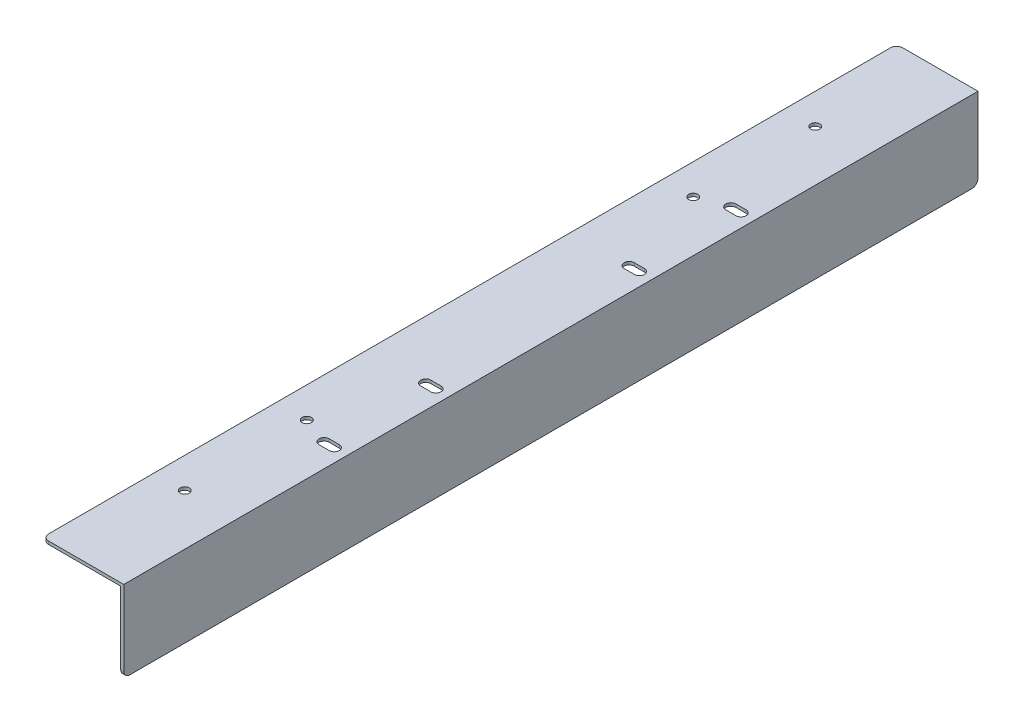
from build123d import *

# Parameters (mm, degrees)
SKETCH_1_W          = 420
SKETCH_1_H          = 40
EXTRUDE_1_DEPTH     = 1.5
SKETCH_2_W          = 420
SKETCH_2_H          = 1.5
EXTRUDE_2_DEPTH     = 40
FILLET_1_R          = 3
SKETCH_3_R          = 2.25
CUT_EXTRUDE_1_DEPTH = 10
SKETCH_6_R          = 2.25
CUT_EXTRUDE_2_DEPTH = 10
CUT_EXTRUDE_3_DEPTH = 218.214755484
CUT_EXTRUDE_4_DEPTH = 218.214755484


with BuildPart() as part:
    # 草图1 → 凸台-拉伸1 (new body)
    with BuildSketch(Plane(origin=(0, 0, 0), x_dir=(0, 0, -1), z_dir=(1, 0, 0))):
        Rectangle(SKETCH_1_W, SKETCH_1_H)
    extrude(amount=EXTRUDE_1_DEPTH)

    # 草图2 → 凸台-拉伸2 (add)
    with BuildSketch(Plane(origin=(1.5, 0, 0), x_dir=(0, 0, -1), z_dir=(1, 0, 0))):
        with Locations((0, 19.25)):
            Rectangle(SKETCH_2_W, SKETCH_2_H)
    extrude(amount=-EXTRUDE_2_DEPTH)

    # 圆角1
    fillet_1_edges = [part.edges().sort_by_distance(p)[0] for p in [
        (-38.5, 19.25, 210),
        (-38.5, 19.25, -210),
        (0.75, -20, -210),
        (0.75, -20, 210),
    ]]
    fillet(fillet_1_edges, radius=FILLET_1_R)

    # 草图3 → 切除-拉伸1 (cut)
    with BuildSketch(Plane(origin=(0, 20, 0), x_dir=(1, 0, 0), z_dir=(0, 1, 0))):
        with Locations(Location((-23.5, -95, 0), (0, 0, 270))):
            Circle(SKETCH_3_R)
        with Locations(Location((-23.5, 95, 0), (0, 0, 90))):
            Circle(SKETCH_3_R)
    extrude(amount=-CUT_EXTRUDE_1_DEPTH, mode=Mode.SUBTRACT)

    # 草图6 → 切除-拉伸2 (cut)
    with BuildSketch(Plane.XZ.offset(-18.5)):
        with Locations(Location((-23.5, -155, 0), (0, 0, 270))):
            Circle(SKETCH_6_R)
        with Locations(Location((-23.5, 155, 0), (0, 0, 270))):
            Circle(SKETCH_6_R)
    extrude(amount=-CUT_EXTRUDE_2_DEPTH, mode=Mode.SUBTRACT)

    # 草图7 → 切除-拉伸3 (cut, through all)
    with BuildSketch(Plane(origin=(0, 20, 0), x_dir=(1, 0, 0), z_dir=(0, 1, 0))):
        with BuildLine():
            Line((-10, -97.5), (-5, -97.5))
            ThreePointArc((-5, -97.5), (-2.5, -100), (-5, -102.5))
            Line((-5, -102.5), (-10, -102.5))
            ThreePointArc((-10, -102.5), (-12.5, -100), (-10, -97.5))
        make_face()
        with BuildLine():
            Line((-5, 47.5), (-10, 47.5))
            ThreePointArc((-10, 47.5), (-12.5, 50), (-10, 52.5))
            Line((-10, 52.5), (-5, 52.5))
            ThreePointArc((-5, 52.5), (-2.5, 50), (-5, 47.5))
        make_face()
    extrude(amount=-CUT_EXTRUDE_3_DEPTH, mode=Mode.SUBTRACT)

    # 草图9 → 切除-拉伸4 (cut, through all)
    with BuildSketch(Plane(origin=(0, 20, 0), x_dir=(1, 0, 0), z_dir=(0, 1, 0))):
        with BuildLine():
            Line((-5, -52.5), (-10, -52.5))
            ThreePointArc((-10, -52.5), (-12.5, -50), (-10, -47.5))
            Line((-10, -47.5), (-5, -47.5))
            ThreePointArc((-5, -47.5), (-2.5, -50), (-5, -52.5))
        make_face()
        with BuildLine():
            Line((-5, 97.5), (-10, 97.5))
            ThreePointArc((-10, 97.5), (-12.5, 100), (-10, 102.5))
            Line((-10, 102.5), (-5, 102.5))
            ThreePointArc((-5, 102.5), (-2.5, 100), (-5, 97.5))
        make_face()
    extrude(amount=-CUT_EXTRUDE_4_DEPTH, mode=Mode.SUBTRACT)


solid = part.part
